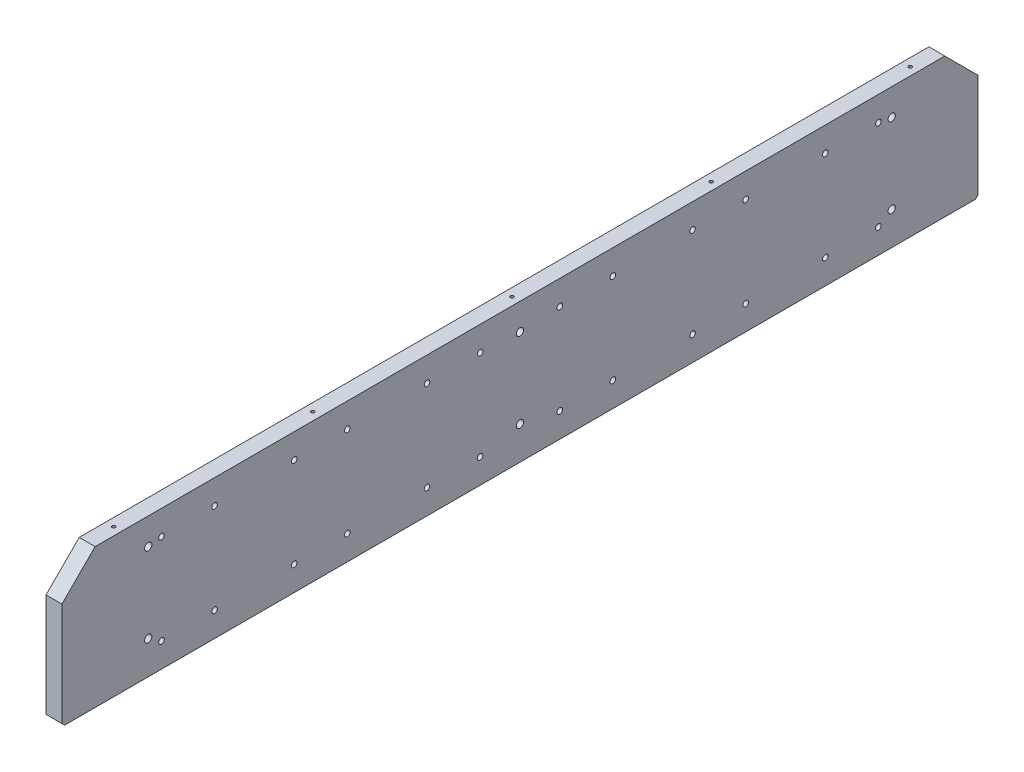
from build123d import *

# Parameters (mm, degrees)
SKETCH_1_W                = 690
SKETCH_1_H                = 105
EXTRUDE_1_DEPTH           = 6
CHAMFER_1_SIZE            = 2
CHAMFER_2_SIZE            = 25
HOLE_WIZARD_M6_1_D        = 5
HOLE_WIZARD_M6_1_DEPTH    = 15
HOLE_WIZARD_M6_1_TIP      = 1.502151548
HOLE_WIZARD_1_D           = 5.5
HOLE_WIZARD_1_CBORE_D     = 10
HOLE_WIZARD_1_CBORE_DEPTH = 5.7
HOLE_WIZARD_M5_1_D        = 4.2
HOLE_WIZARD_M3_2_D        = 2.5
HOLE_WIZARD_M3_2_DEPTH    = 7.5
HOLE_WIZARD_M3_2_TIP      = 0.751075774


with BuildPart() as part:
    # 草图1 → 凸台-拉伸1 (new, symmetric)
    with BuildSketch(Plane(origin=(0, 0, 0), x_dir=(0, 0, -1), z_dir=(1, 0, 0))):
        Rectangle(SKETCH_1_W, SKETCH_1_H)
    extrude(amount=EXTRUDE_1_DEPTH, both=True)

    # 倒角1
    chamfer_1_edges = [part.edges().sort_by_distance(p)[0] for p in [
        (0, -52.5, -345),
        (0, -52.5, 345),
    ]]
    chamfer(chamfer_1_edges, length=CHAMFER_1_SIZE)

    # 倒角2
    chamfer_2_edges = [part.edges().sort_by_distance(p)[0] for p in [
        (0, 52.5, 345),
        (0, 52.5, -345),
    ]]
    chamfer(chamfer_2_edges, length=CHAMFER_2_SIZE)

    # M6 螺纹孔1
    with Locations(Plane(origin=(0, -52.5, 0), x_dir=(-1, 0, 0), z_dir=(0, -1, 0))):
        with Locations((0, -300), (0, -150), (0, 0), (0, 150), (0, 300)):
            Hole(HOLE_WIZARD_M6_1_D / 2, depth=HOLE_WIZARD_M6_1_DEPTH)
            with Locations((0, 0, -(HOLE_WIZARD_M6_1_DEPTH + HOLE_WIZARD_M6_1_TIP / 2))):  # 118° drill point
                Cone(0, HOLE_WIZARD_M6_1_D / 2, HOLE_WIZARD_M6_1_TIP, mode=Mode.SUBTRACT)

    # 打孔尺寸(%根据)内六角圆柱头螺钉的类型1 (through all)
    with Locations(Plane.ZY.offset(6)):
        with Locations((280, 32.5), (280, -27.5), (0, 32.5), (0, -27.5), (-280, 32.5), (-280, -27.5)):
            CounterBoreHole(HOLE_WIZARD_1_D / 2, HOLE_WIZARD_1_CBORE_D / 2, HOLE_WIZARD_1_CBORE_DEPTH)

    # M5 螺纹孔1 (through all)
    with Locations(Plane.ZY.offset(6)):
        with Locations((270, 34), (270, -34), (170, 34), (170, -34), (70, 34), (70, -34), (-30, 34), (-30, -34), (-130, 34), (-130, -34), (130, -34), (130, 34), (30, -34), (30, 34), (-70, -34), (-70, 34), (-170, -34), (-170, 34), (-270, -34), (-270, 34), (-230, 34), (-230, -34), (230, -34), (230, 34)):
            Hole(HOLE_WIZARD_M5_1_D / 2)

    # M3 螺纹孔2
    with Locations(Plane(origin=(0, 52.5, 0), x_dir=(1, 0, 0), z_dir=(0, 1, 0))):
        with Locations((0, -300), (0, -150), (0, 0), (0, 150), (0, 300)):
            Hole(HOLE_WIZARD_M3_2_D / 2, depth=HOLE_WIZARD_M3_2_DEPTH)
            with Locations((0, 0, -(HOLE_WIZARD_M3_2_DEPTH + HOLE_WIZARD_M3_2_TIP / 2))):  # 118° drill point
                Cone(0, HOLE_WIZARD_M3_2_D / 2, HOLE_WIZARD_M3_2_TIP, mode=Mode.SUBTRACT)


solid = part.part
